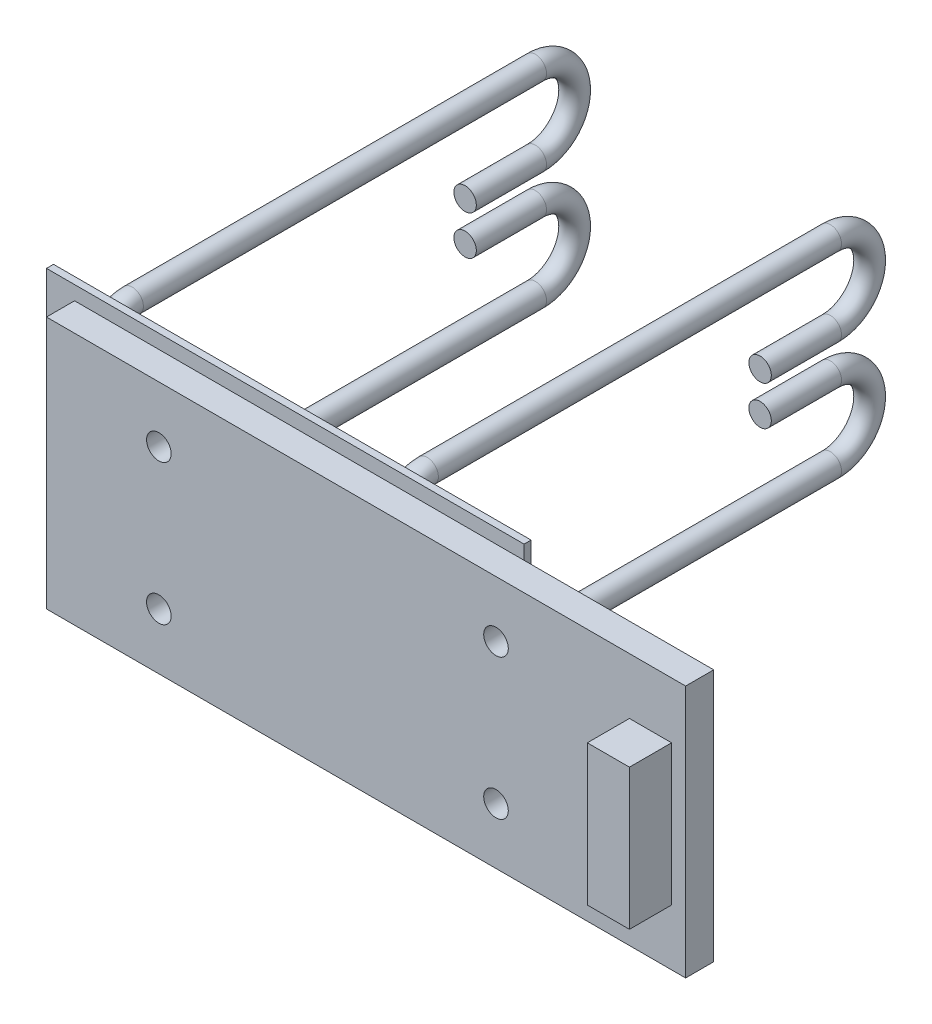
SolidWorks part; units mm, degrees
material "A3"
ref_plane "前视基准面" through (0, 0, 0) normal (0, 0, 1) x (1, 0, 0)
ref_plane "上视基准面" through (0, 0, 0) normal (0, 1, 0) x (1, 0, 0)
ref_plane "右视基准面" through (0, 0, 0) normal (1, 0, 0) x (0, 0, -1)
sketch "草图1" plane through (0, 0, 0) normal (0, 0, 1) x (1, 0, 0)
  line L1 (-227.5, -90) -> (227.5, -90)
  line L2 (-227.5, -90) -> (-227.5, 90)
  line L3 (-227.5, 90) -> (227.5, 90)
  line L4 (227.5, -90) -> (227.5, 90)
  line L5 (-227.5, -90) -> (227.5, 90) construction
  line L6 (-227.5, 90) -> (227.5, -90) construction
  point P0 (0, 0)
  dimension "D1" = 180
  dimension "D2" = 455
extrude "凸台-拉伸1" add sketch "草图1" along normal blind 20
sketch "草图2" plane through (0, 0, 20) normal (0, 0, 1) x (1, 0, 0)
  line L0 (-227.5, 90) -> (-227.5, -90) construction
  line L1 (217.5, -50) -> (187.5, -50)
  line L2 (217.5, -50) -> (217.5, 50)
  line L3 (217.5, 50) -> (187.5, 50)
  line L4 (187.5, -50) -> (187.5, 50)
  line L5 (217.5, -50) -> (187.5, 50) construction
  line L6 (217.5, 50) -> (187.5, -50) construction
  point P0 (202.5, 0)
  dimension "D1" = 100
  dimension "D2" = 30
  dimension "D3" = 415
extrude "凸台-拉伸2" add sketch "草图2" along normal blind 30 separate body
sketch "草图3" plane through (0, 0, 0) normal (0, 0, -1) x (-1, 0, 0)
  line L0 (227.5, 90) -> (227.5, -90) construction
  line L1 (-92.5, -100) -> (247.5, -100)
  line L2 (-92.5, -100) -> (-92.5, 100)
  line L3 (-92.5, 100) -> (247.5, 100)
  line L4 (247.5, -100) -> (247.5, 100)
  line L5 (-92.5, -100) -> (247.5, 100) construction
  line L6 (-92.5, 100) -> (247.5, -100) construction
  point P0 (77.5, 0)
  dimension "D1" = 200
  dimension "D2" = 340
  dimension "D3" = 20
extrude "凸台-拉伸3" add sketch "草图3" along normal blind 5 separate body
sketch "草图4" plane through (-227.5, 0, 0) normal (-1, 0, 0) x (0, 0, 1)
  line L0 (0, 0) -> (-68.5253, 0) construction
  line L1 (-13, -42) -> (-13, 42)
  line L2 (-41, 70) -> (-328, 70)
  line L3 (-328, 70) -> (-328, 14) construction
  line L4 (-328, 14) -> (-278, 14)
  line L5 (-5, -100) -> (-5, 100) construction
  line L6 (-328, -70) -> (-328, -14) construction
  line L7 (-328, -14) -> (-278, -14)
  line L8 (-41, -70) -> (-328, -70)
  arc A0 (-328, 70) -> (-328, 14) centre (-328, 42) ccw
  arc A1 (-13, 42) -> (-41, 70) centre (-41, 42) ccw
  arc A2 (-13, -42) -> (-41, -70) centre (-41, -42) cw
  arc A3 (-328, -70) -> (-328, -14) centre (-328, -42) cw
  point P20 (-13, 0)
  dimension "D1" = 8
  dimension "D4" = 28
  dimension "D6" = 28
  dimension "D2" = 140
  dimension "D3" = 50
  dimension "D5" = 323
sweep "扫描1" add path "草图4" circular profile diameter 16 parameters "D3"=16
pattern_linear "阵列(线性)1" count 2 spacing 210 along (1, 0, 0) of bodies 109
hole_wizard "M20 螺纹孔1" positions "草图6" profile "草图7" tap size "M20" standard "GB"
sketch "草图6" plane through (0, 0, -5) normal (0, 0, -1) x (-1, 0, 0)
  line L0 (-227.5, -90) -> (-227.5, 90) construction
  line L1 (-92.5, -50) -> (147.5, -50) construction
  line L2 (-92.5, -50) -> (-92.5, 50) construction
  point P0 (-92.5, -50)
  point P11 (147.5, -50)
  point P12 (147.5, 50)
  point P13 (-92.5, 50)
  dimension "D1" = 50
  dimension "D2" = 135
  dimension "D5" = 240
  dimension "D6" = 100
  dimension "D3" = 2
  dimension "D4" = 2
sketch "草图7" plane through (92.5, -50, -5) normal (1, 0, 0) x (0, 1, 0)
  line L0 (0, 0) -> (0, 57.7575)
  line L1 (0, 57.7575) -> (8.75, 52.5)
  line L2 (8.75, 52.5) -> (8.75, 0)
  line L5 (8.75, 0) -> (0, 0)
  line L10 (0, 57.7575) -> (-8.75, 52.5) construction
  line L11 (0, -6.35) -> (0, 107.95) construction
  dimension "螺纹孔钻头直径" = 17.5
  dimension "螺纹孔钻头深度" = 52.5
  dimension "导头角度" = 118
cosmetic thread "孔螺蚊线1" parameters "D1"=40, "D2"=20
cosmetic thread "孔螺蚊线2" parameters "D1"=40, "D2"=20
cosmetic thread "孔螺蚊线3" parameters "D1"=40, "D2"=20
cosmetic thread "孔螺蚊线4" parameters "D1"=40, "D2"=20
sketch "草图8" plane through (0, 0, -5) normal (0, 0, -1) x (-1, 0, 0)
  line L0 (247.5, -100) -> (247.5, 100) construction
  line L1 (207.5, -70) -> (117.5, -70)
  line L2 (207.5, -70) -> (207.5, 70)
  line L3 (207.5, 70) -> (117.5, 70)
  line L4 (117.5, -70) -> (117.5, 70)
  line L5 (207.5, -70) -> (117.5, 70) construction
  line L6 (207.5, 70) -> (117.5, -70) construction
  point P0 (162.5, 0)
  dimension "D1" = 140
  dimension "D2" = 90
  dimension "D3" = 40
extrude "凸台-拉伸4" add sketch "草图8" along normal blind 3 separate body
pattern_linear "阵列(线性)2" count 2 spacing 240 along (1, 0, 0) of bodies 113
